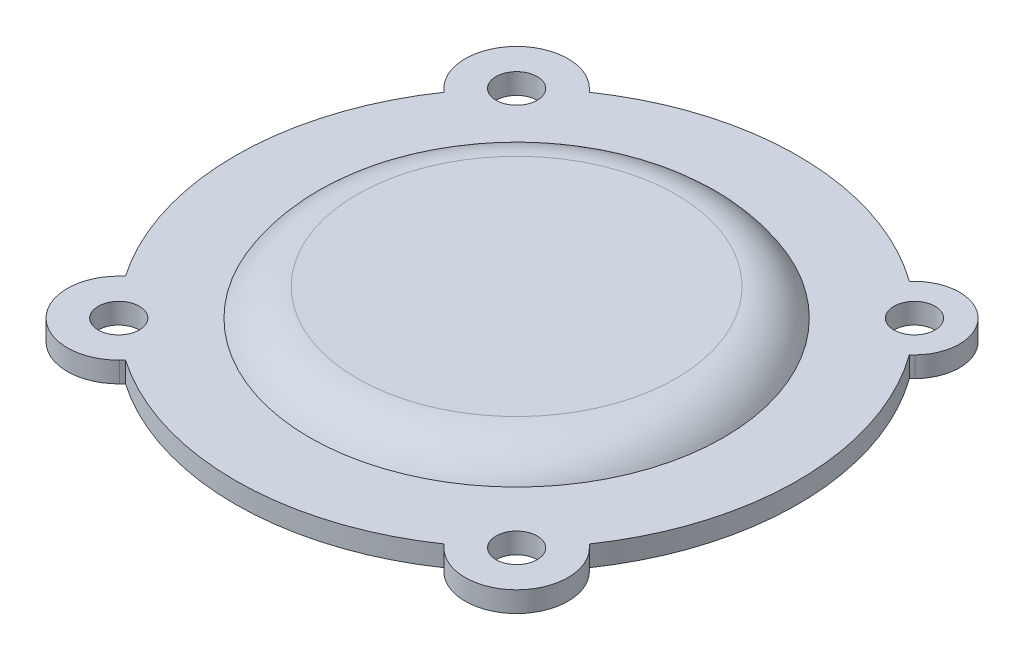
from build123d import *

# Parameters (mm, degrees)
EXTRUDE_START       = -3
SKETCH_2_R          = 35.459459581
EXTRUDE_1_DEPTH     = 3
SKETCH_4_R          = 3
CUT_EXTRUDE_1_DEPTH = 59.532042507


with BuildPart() as part:
    # 草图1 → 旋转1 (revolve)
    with BuildSketch(Plane(origin=(0, 0, 0), x_dir=(0, 0, -1), z_dir=(1, 0, 0)), mode=Mode.PRIVATE) as revolve_1_sk:
        with BuildLine():
            Line((0, 12), (23.23298563, 12))
            ThreePointArc((23.23298563, 12), (27.23298563, 10.92820323), (30.16118886, 8))
            Line((30.16118886, 8), (41, 8))
            Line((41, 8), (41, 5))
            Line((41, 5), (31, 5))
            Line((31, 5), (31, 0))
            Line((31, 0), (28, 0))
            Line((28, 0), (27.172216642, 4.694592711))
            ThreePointArc((27.172216642, 4.694592711), (25.804136068, 7.064177772), (23.23298563, 8))
            Line((23.23298563, 8), (21.200995797, 8))
            Line((21.200995797, 8), (0, 8))
            Line((0, 8), (0, 12))
        make_face()
    revolve(revolve_1_sk.sketch.rotate(Axis((0, 53.940866142, 0), (0, -1, 0)), 180), axis=Axis((0, 53.940866142, 0), (0, -1, 0)))

    # 草图2 → 凸台-拉伸1 (add)
    with BuildSketch(Plane(origin=(0, 8, 0), x_dir=(1, 0, 0), z_dir=(0, 1, 0)).offset(EXTRUDE_START)):
        with BuildLine():
            Line((-34.294678434, 23.688076669), (-33.80549374, 23.198892063))
            ThreePointArc((-33.80549374, 23.198892063), (-40.999999826, -0.003774812), (-33.801221389, -23.205116518))
            Line((-33.801221389, -23.205116518), (-34.233536486, -23.627631697))
            ThreePointArc((-34.233536486, -23.627631697), (-34.294678888, -34.294678888), (-23.627631697, -34.233536486))
            Line((-23.627631697, -34.233536486), (-23.205116518, -33.801221389))
            ThreePointArc((-23.205116518, -33.801221389), (-0.003771108, -40.999999827), (23.198898172, -33.805489549))
            Line((23.198898172, -33.805489549), (23.680662822, -34.287254142))
            ThreePointArc((23.680662822, -34.287254142), (34.291151869, -34.298203544), (34.294310993, -23.687709319))
            Line((34.294310993, -23.687709319), (33.805466141, -23.198932281))
            ThreePointArc((33.805466141, -23.198932281), (40.997262845, 0.473750181), (33.260352966, 23.973921676))
            Line((33.260352966, 23.973921676), (33.682868145, 24.406236773))
            ThreePointArc((33.682868145, 24.406236773), (33.629998505, 33.629998505), (24.406236773, 33.682868145))
            Line((24.406236773, 33.682868145), (23.973921676, 33.260352966))
            ThreePointArc((23.973921676, 33.260352966), (0.470906346, 40.997295609), (-23.203621987, 33.802247362))
            Line((-23.203621987, 33.802247362), (-23.642860481, 34.249073393))
            ThreePointArc((-23.642860481, 34.249073393), (-34.27192479, 34.317335821), (-34.294678434, 23.688076669))
        make_face()
        Circle(SKETCH_2_R, mode=Mode.SUBTRACT)
    extrude(amount=EXTRUDE_1_DEPTH)

    # 草图4 → 切除-拉伸1 (cut, through all)
    with BuildSketch(Plane(origin=(0, 8, 0), x_dir=(1, 0, 0), z_dir=(0, 1, 0))):
        with Locations(Location((-28.991378029, 28.991378029, 0), (0, 0, 270))):
            Circle(SKETCH_4_R)
        with Locations(Location((28.991378029, 28.991378029, 0), (0, 0, 270))):
            Circle(SKETCH_4_R)
        with Locations(Location((28.991378029, -28.991378029, 0), (0, 0, 270))):
            Circle(SKETCH_4_R)
        with Locations(Location((-28.991378029, -28.991378029, 0), (0, 0, 270))):
            Circle(SKETCH_4_R)
    extrude(amount=-CUT_EXTRUDE_1_DEPTH, mode=Mode.SUBTRACT)


solid = part.part
